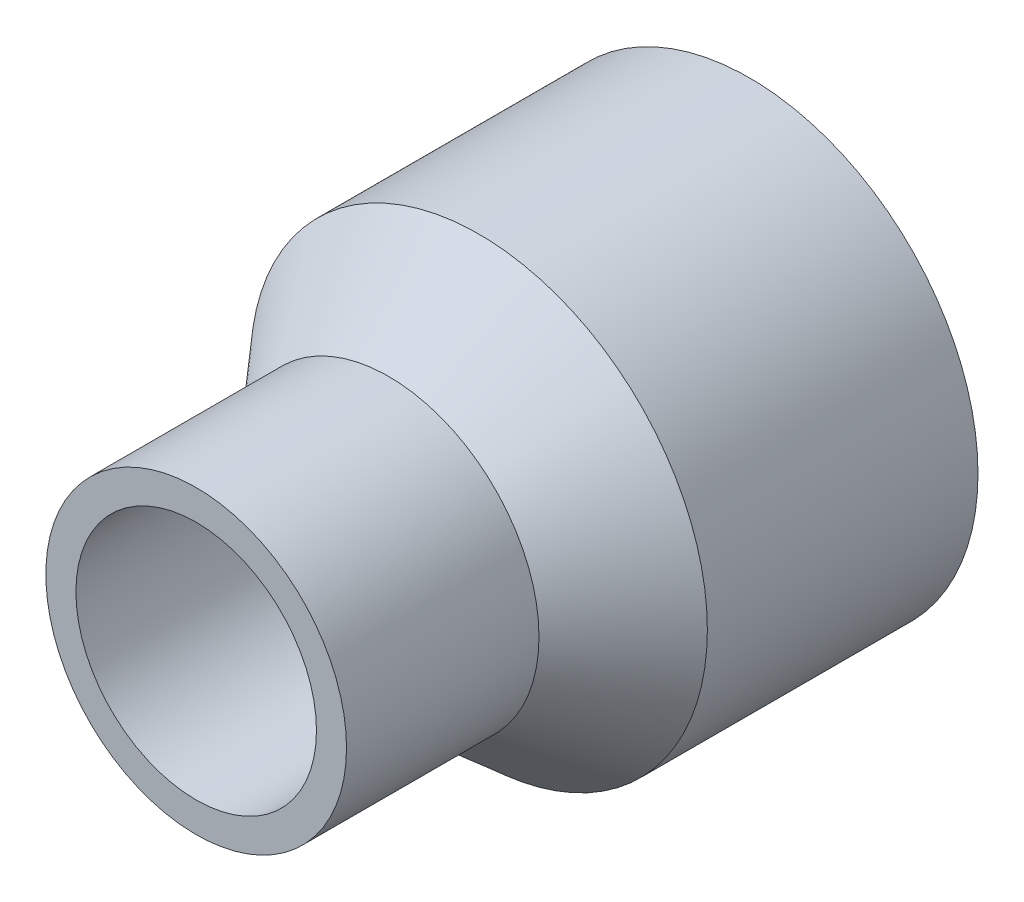
from build123d import *


with BuildPart() as part:
    # 草图1 → 旋转1 (revolve)
    with BuildSketch(Plane(origin=(0, 0, 0), x_dir=(0, 0, -1), z_dir=(1, 0, 0)), mode=Mode.PRIVATE) as revolve_1_sk:
        Polygon((53.611052376, 10), (69.611052376, 10), (77.111052376, 16), (99.611052376, 16), (99.611052376, 19), (77.111052376, 19), (69.611052376, 12.5), (53.611052376, 12.5), align=None)
    revolve(revolve_1_sk.sketch.rotate(Axis((0, 0, 0), (0, 0, -1)), 90), axis=Axis((0, 0, 0), (0, 0, -1)))


solid = part.part
